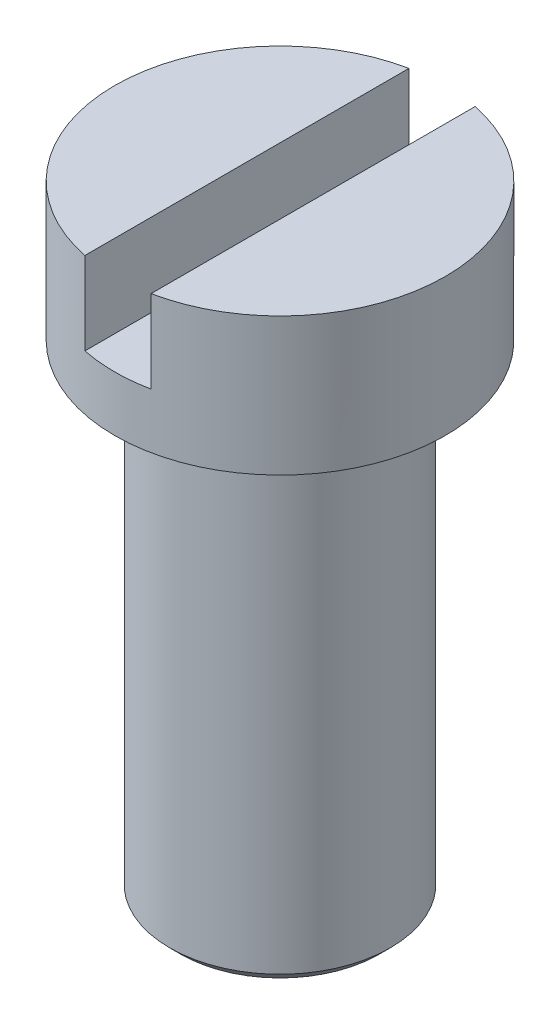
SolidWorks part; units mm, degrees
ref_plane "前视基准面" through (0, 0, 0) normal (0, 0, 1) x (1, 0, 0)
ref_plane "上视基准面" through (0, 0, 0) normal (0, 1, 0) x (1, 0, 0)
ref_plane "右视基准面" through (0, 0, 0) normal (1, 0, 0) x (0, 0, -1)
other "Configuration Table"
sketch "草图1" plane through (0, 0, 0) normal (0, 1, 0) x (1, 0, 0)
  circle A0 centre (0, 0) radius 20
  dimension "D1" = 40
extrude "凸台-拉伸1" add sketch "草图1" along normal mid plane 100 contours A0
sketch "草图2" plane through (0, 50, 0) normal (0, 1, 0) x (1, 0, 0)
  circle A0 centre (0, 0) radius 30
  dimension "D1" = 60
extrude "凸台-拉伸2" add sketch "草图2" along normal mid plane 25 contours A0
chamfer "倒角1" distance 2 angle 45 1 edges at (0, -50, 20)
sketch "草图3" plane through (0, 62.5, 0) normal (0, 1, 0) x (1, 0, 0)
  line L1 (-6, -38.7492) -> (6, -38.7492)
  line L2 (-6, -38.7492) -> (-6, 38.7492)
  line L3 (-6, 38.7492) -> (6, 38.7492)
  line L4 (6, -38.7492) -> (6, 38.7492)
  line L5 (-6, -38.7492) -> (6, 38.7492) construction
  line L6 (-6, 38.7492) -> (6, -38.7492) construction
  point P0 (0, 0)
  dimension "D1" = 12
extrude "切除-拉伸1" cut sketch "草图3" against normal blind 15 contours L4 L3 L2 L1
